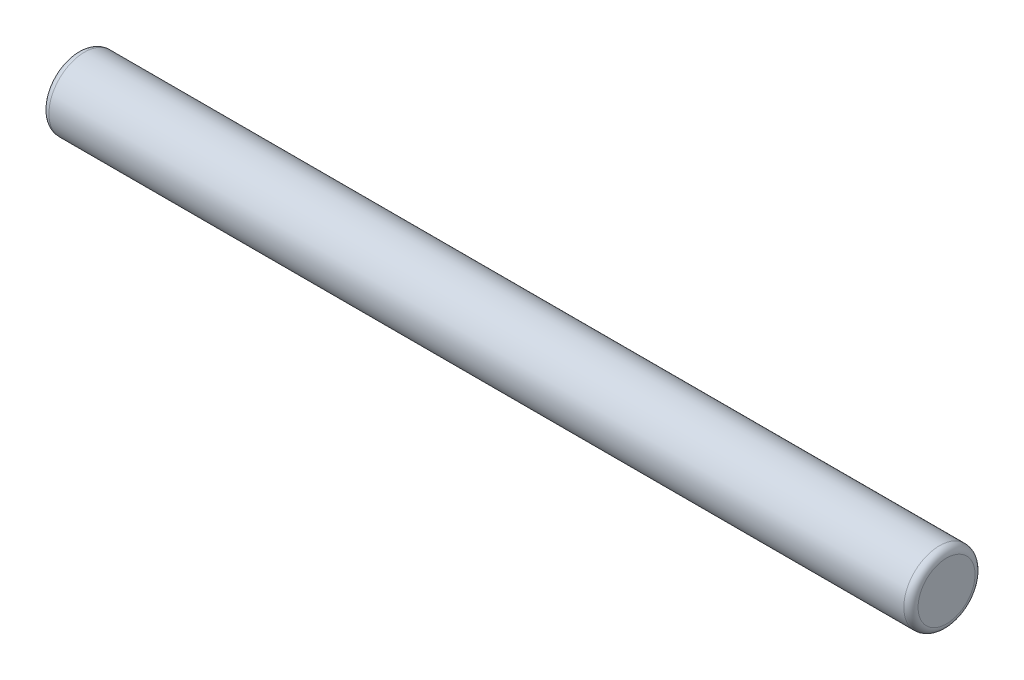
SolidWorks part; units mm, degrees
material "不锈钢304"
ref_plane "前视基准面" through (0, 0, 0) normal (0, 0, 1) x (1, 0, 0)
ref_plane "上视基准面" through (0, 0, 0) normal (0, 1, 0) x (1, 0, 0)
ref_plane "右视基准面" through (0, 0, 0) normal (1, 0, 0) x (0, 0, -1)
sketch "草图1" plane through (0, 0, 0) normal (1, 0, 0) x (0, 0, -1)
  circle A0 centre (0, 0) radius 1
  dimension "D1" = 2
extrude "凸台-拉伸1" add sketch "草图1" along normal mid plane 24.4
fillet "圆角1" radius 0.2 2 edges at (12.2, 0, -1) (-12.2, 0, -1)
